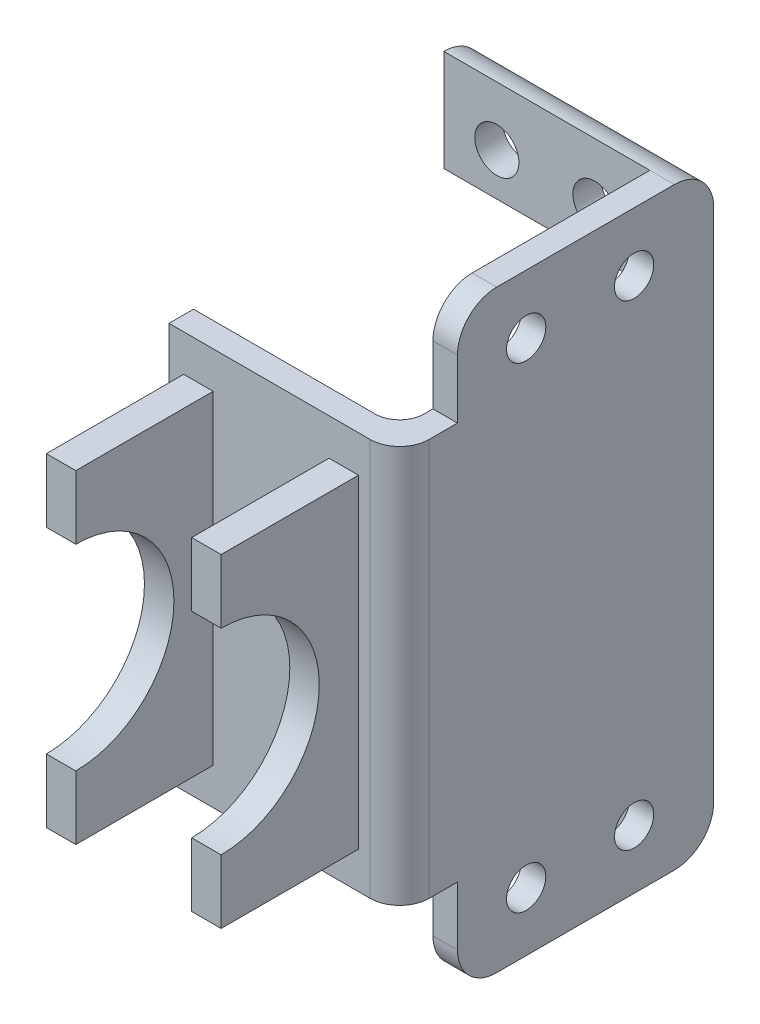
from build123d import *

# Parameters (mm, degrees)
SKETCH2_W           = 21
SKETCH2_H           = 40.5
BOSS_EXTRUDE1_DEPTH = 2.5
SKETCH3_W           = 3
SKETCH3_H           = 33
BOSS_EXTRUDE2_DEPTH = 14
SKETCH4_R           = 10
CUT_EXTRUDE1_DEPTH  = 40.501767279
BOSS_EXTRUDE3_DEPTH = 20.25
FILLET1_R           = 3
FILLET2_R           = 2.5
BOSS_EXTRUDE4_DEPTH = 2.5
SKETCH7_R           = 2
CUT_EXTRUDE2_DEPTH  = 56.162442887
BOSS_EXTRUDE5_DEPTH = 21
SKETCH10_R          = 2.25
CUT_EXTRUDE3_DEPTH  = 21


with BuildPart() as part:
    # Sketch2 → Boss-Extrude1 (new body)
    with BuildSketch(Plane.XY):
        with Locations((0.095633845, -10.004131531)):
            Rectangle(SKETCH2_W, SKETCH2_H)
    extrude(amount=BOSS_EXTRUDE1_DEPTH)

    # Sketch3 → Boss-Extrude2 (add)
    with BuildSketch(Plane.XY.offset(2.5)):
        with Locations((-7.404366155, -10.004131531)):
            Rectangle(SKETCH3_W, SKETCH3_H)
        with Locations((7.404366155, -10.004131531)):
            Rectangle(SKETCH3_W, SKETCH3_H)
    extrude(amount=BOSS_EXTRUDE2_DEPTH)

    # Sketch4 → Cut-Extrude1 (cut, through all)
    with BuildSketch(Plane(origin=(8.904366155, 0, 0), x_dir=(0, 0, -1), z_dir=(1, 0, 0))):
        with Locations((-16.5, -10.004131531)):
            Circle(SKETCH4_R)
    extrude(amount=-CUT_EXTRUDE1_DEPTH, mode=Mode.SUBTRACT)

    # Sketch5 → Boss-Extrude3 (add, symmetric)
    with BuildSketch(Plane(origin=(0, -10.004131531, 0), x_dir=(1, 0, 0), z_dir=(0, 1, 0))):
        Polygon((10.595633845, 0), (10.595633845, 29.5), (13.095633845, 29.5), (13.095633845, -2.5), (10.595633845, -2.5), align=None)
    extrude(amount=BOSS_EXTRUDE3_DEPTH, both=True)

    # Fillet1
    fillet1_edges = [part.edges().sort_by_distance(p)[0] for p in [
        (13.095633845, -10.004131531, 2.5),
    ]]
    fillet(fillet1_edges, radius=FILLET1_R)

    # Fillet2
    fillet2_edges = [part.edges().sort_by_distance(p)[0] for p in [
        (10.595633845, -10.004131531, 0),
    ]]
    fillet(fillet2_edges, radius=FILLET2_R)

    # Sketch6 → Boss-Extrude4 (add)
    with BuildSketch(Plane(origin=(13.095633845, 0, 0), x_dir=(0, 0, -1), z_dir=(1, 0, 0))):
        with BuildLine():
            Line((29.5, -30.254131531), (29.5, -36.254131531))
            ThreePointArc((29.5, -36.254131531), (28.328427125, -39.082558656), (25.5, -40.254131531))
            Line((25.5, -40.254131531), (7.39536549, -40.254131531))
            ThreePointArc((7.39536549, -40.254131531), (4.566938365, -39.082558656), (3.39536549, -36.254131531))
            Line((3.39536549, -36.254131531), (3.39536549, -30.254131531))
            Line((3.39536549, -30.254131531), (29.5, -30.254131531))
        make_face()
        with BuildLine():
            Line((3.39536549, 10.245868469), (29.5, 10.245868469))
            Line((29.5, 10.245868469), (29.5, 16.245868469))
            ThreePointArc((29.5, 16.245868469), (28.328427125, 19.074295594), (25.5, 20.245868469))
            Line((25.5, 20.245868469), (7.39536549, 20.245868469))
            ThreePointArc((7.39536549, 20.245868469), (4.566938365, 19.074295594), (3.39536549, 16.245868469))
            Line((3.39536549, 16.245868469), (3.39536549, 10.245868469))
        make_face()
    extrude(amount=-BOSS_EXTRUDE4_DEPTH)

    # Sketch7 → Cut-Extrude2 (cut, through all)
    with BuildSketch(Plane(origin=(13.095633845, 0, 0), x_dir=(0, 0, -1), z_dir=(1, 0, 0))):
        with Locations((21.39536549, -34.254131531)):
            Circle(SKETCH7_R)
        with Locations((10.39536549, -34.254131531)):
            Circle(SKETCH7_R)
        with Locations((10.39536549, 14.245868469)):
            Circle(SKETCH7_R)
        with Locations((21.39536549, 14.245868469)):
            Circle(SKETCH7_R)
    extrude(amount=-CUT_EXTRUDE2_DEPTH, mode=Mode.SUBTRACT)

    # Sketch9 → Boss-Extrude5 (add)
    with BuildSketch(Plane.ZY.offset(-10.595633845)):
        with BuildLine():
            Line((-28.328427125, -39.082558656), (-28.328427125, -29.914909502))
            Line((-28.328427125, -29.914909502), (-25.5, -29.914909502))
            Line((-25.5, -29.914909502), (-25.5, -40.254131531))
            ThreePointArc((-25.5, -40.254131531), (-27.030733729, -39.949649661), (-28.328427125, -39.082558656))
        make_face()
    boss_extrude5 = extrude(amount=BOSS_EXTRUDE5_DEPTH)

    # Mirror1: Boss-Extrude5 across plane
    add(boss_extrude5.mirror(Plane.ZX.offset(-10.004131531)))

    # Sketch10 → Cut-Extrude3 (cut)
    with BuildSketch(Plane(origin=(0, 0, -28.328427125), x_dir=(-1, 0, 0), z_dir=(0, 0, -1))):
        with Locations(Location((-5, -34.25, 0), (0, 0, 90))):
            Circle(SKETCH10_R)
        with Locations(Location((5, -34.25, 0), (0, 0, 90))):
            Circle(SKETCH10_R)
    cut_extrude3 = extrude(amount=-CUT_EXTRUDE3_DEPTH, mode=Mode.SUBTRACT)

    # Mirror2: Cut-Extrude3 across plane
    add(cut_extrude3.mirror(Plane.ZX.offset(-10.004131531)), mode=Mode.SUBTRACT)


solid = part.part
